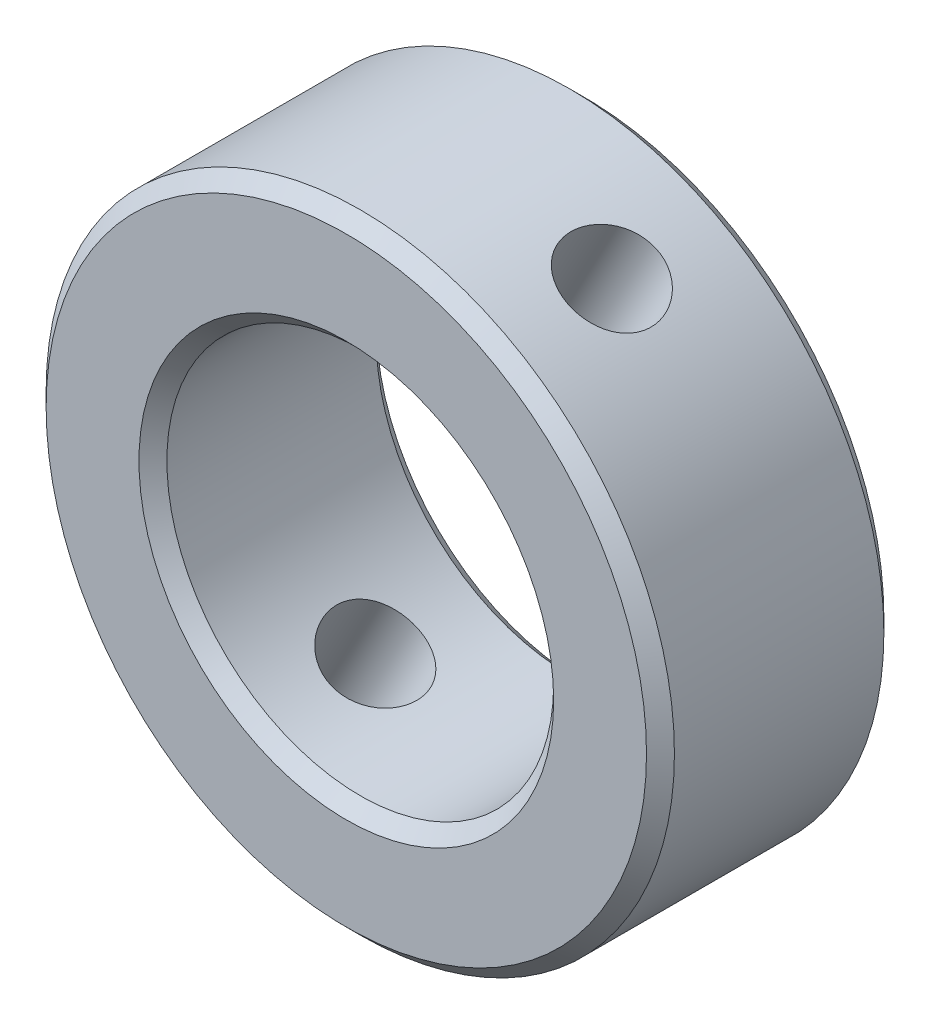
SolidWorks part; units mm, degrees
ref_plane "Front Plane" through (0, 0, 0) normal (0, 0, 1) x (1, 0, 0)
ref_plane "Top Plane" through (0, 0, 0) normal (0, 1, 0) x (1, 0, 0)
ref_plane "Right Plane" through (0, 0, 0) normal (1, 0, 0) x (0, 0, -1)
sketch "Sketch1" plane through (0, 0, 0) normal (0, 0, 1) x (1, 0, 0)
  circle A0 centre (0, 0) radius 27.7
  circle A1 centre (0, 0) radius 45
  dimension "D1" = 55.4
  dimension "D2" = 90
extrude "Boss-Extrude1" add sketch "Sketch1" along normal blind 34
hole_wizard "Ø13.0 (13) Diameter Hole1" positions "3DSketch1" profile "Sketch3" hole size "Ø13.0" standard "GB" end condition through all
sketch3d "3DSketch1"
  point P0 (21.1311, 39.7301, 17)
  dimension "D1" = 17
sketch "Sketch3" plane through (21.1311, 39.7301, 17) normal (0, 0, 1) x (-0.8829, 0.4696, 0)
  line L0 (0, 0) -> (0, 105.8611)
  line L1 (0, 105.8611) -> (6.5, 105.8611)
  line L2 (6.5, 105.8611) -> (6.5, 0)
  line L5 (6.5, 0) -> (0, 0)
  line L11 (0, -6.35) -> (0, 107.95) construction
  dimension "通孔孔直径" = 13
  dimension "通孔孔深度" = 105.8611
chamfer "Chamfer1" distance 2 angle 45 4 edges at (45, 0, 0) (27.7, 0, 0) (27.7, 0, 34) (45, 0, 34)
